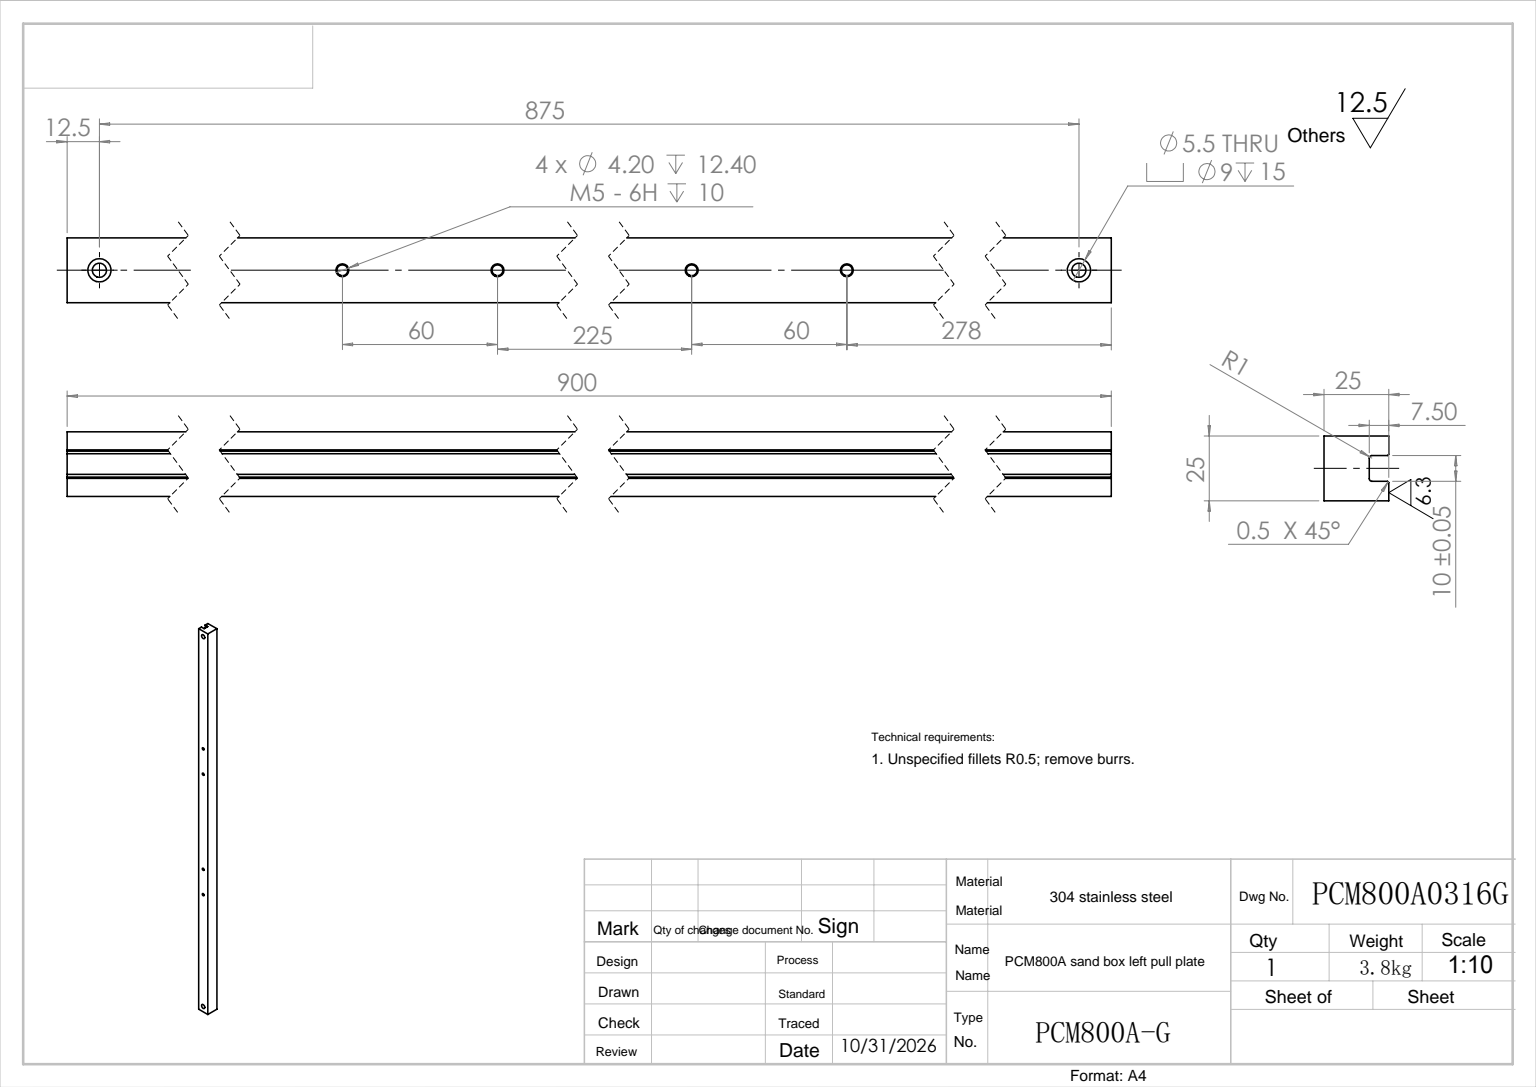
SolidWorks part; units mm, degrees
ref_plane "前视" through (0, 0, 0) normal (0, 0, 1) x (1, 0, 0)
ref_plane "上视" through (0, 0, 0) normal (0, 1, 0) x (1, 0, 0)
ref_plane "右视" through (0, 0, 0) normal (1, 0, 0) x (0, 0, -1)
sketch "草图1" plane through (0, 0, 0) normal (1, 0, 0) x (0, 0, -1)
  line L1 (0, 0) -> (25, 0)
  line L2 (0, 0) -> (0, 900)
  line L3 (0, 900) -> (25, 900)
  line L4 (25, 0) -> (25, 900)
  dimension "D1" = 25
  dimension "D2" = 900
extrude "拉伸1" add sketch "草图1" along normal blind 25
sketch "草图2" plane through (0, 0, 0) normal (0, -1, 0) x (1, 0, 0)
  line L0 (0, 0) -> (0, -25) construction
  line L1 (0, -7.5) -> (6.5, -7.5)
  line L2 (0, -7.5) -> (0, -17.5)
  line L3 (0, -17.5) -> (6.5, -17.5)
  line L4 (7.5, -8.5) -> (7.5, -16.5)
  arc A0 (6.5, -7.5) -> (7.5, -8.5) centre (6.5, -8.5) cw
  arc A1 (6.5, -17.5) -> (7.5, -16.5) centre (6.5, -16.5) ccw
  point P9 (7.5, -7.5)
  point P12 (7.5, -17.5)
  dimension "D4" = 1
  dimension "D1" = 10
  dimension "D2" = 7.5
  dimension "D3" = 7.5
extrude "切除-拉伸1" cut sketch "草图2" against normal through all
chamfer "倒角1" distance 0.5 angle 45 2 edges at (0, 450, -17.5) (0, 450, -7.5)
sketch "草图3" plane through (0, 0, 0) normal (0, 0, 1) x (1, 0, 0)
  line L0 (12.5, 900) -> (12.5, 0) construction
  line L1 (25, 900) -> (0, 900) construction
  line L2 (25, 0) -> (0, 0) construction
  line L3 (12.5, 12.5) -> (25, 12.5) construction
  line L4 (25, 900) -> (25, 0) construction
  line L8 (12.5, 887.5) -> (25, 887.5) construction
  dimension "D1" = 12.5
  dimension "D2" = 12.5
hole_wizard "孔1" positions "3D草图1" profile "草图4" legacy end condition through all
sketch3d "3D草图1"
  line L2 (25, 900, 0) -> (0, 900, 0) construction
  line L3 (25, 900, 0) -> (25, 0, 0) construction
  line L4 (25, 0, 0) -> (0, 0, 0) construction
  point P11 (12.5, 887.5, 0)
  point P13 (12.5, 12.5, 0)
  dimension "D1" = 12.5
  dimension "D2" = 12.5
  dimension "D3" = 12.5
  dimension "D4" = 12.5
sketch "草图4" plane through (12.5, 887.5, 0) normal (1, 0, 0) x (0, -1, 0)
  line L0 (0, 0) -> (0, 25)
  line L1 (0, 25) -> (2.75, 25)
  line L3 (2.75, 25) -> (2.75, 15)
  line L4 (2.75, 15) -> (4.5, 15)
  line L5 (4.5, 15) -> (4.5, 0)
  line L7 (4.5, 0) -> (0, 0)
  line L11 (0, -6.35) -> (0, 107.95) construction
  dimension "籵謂謂眻噤" = 5.5
  dimension "籵謂謂旮僅" = 25
  dimension "翐倛麥芛謂眻噤" = 9
  dimension "翐倛麥芛謂旮僅" = 15
hole_wizard "M5 螺纹孔1" positions "3D草图2" profile "草图5" tap size "M5" standard "GB"
sketch3d "3D草图2"
  line L0 (25, 900, 0) -> (25, 0, 0) construction
  line L1 (25, 900, 0) -> (0, 900, 0) construction
  point P0 (12.5, 622, 0)
  point P2 (12.5, 562, 0)
  dimension "D1" = 12.5
  dimension "D2" = 12.5
  dimension "D3" = 60
  dimension "D4" = 278
sketch "草图5" plane through (12.5, 622, 0) normal (1, 0, 0) x (0, -1, 0)
  line L0 (0, 0) -> (0, 13.6618)
  line L1 (0, 13.6618) -> (2.1, 12.4)
  line L2 (2.1, 12.4) -> (2.1, 10)
  line L3 (2.1, 10) -> (2.5, 10)
  line L4 (2.5, 10) -> (2.5, 0)
  line L5 (2.5, 0) -> (0, 0)
  line L10 (0, 13.6618) -> (-2.1, 12.4) construction
  line L11 (0, -6.35) -> (0, 107.95) construction
  dimension "螺纹孔钻头直径" = 4.2
  dimension "螺纹孔钻头深度" = 12.4
  dimension "螺纹主直径" = 5
  dimension "螺纹深度" = 10
  dimension "导头角度" = 118
pattern_linear "阵列(线性)1" count 2 spacing 285 along (0, -1, 0) of "M5 螺纹孔1"
